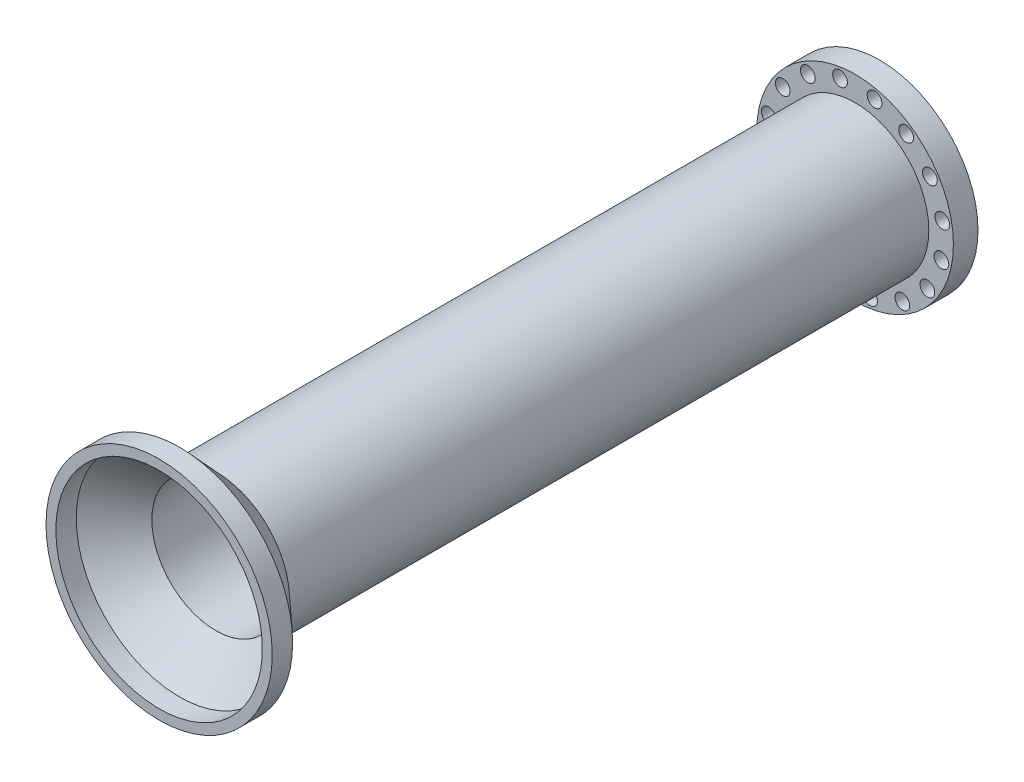
from build123d import *

# Parameters (mm, degrees)
SKETCH1_R               = 20
SKETCH1_R_2             = 15
BOSS_EXTRUDE1_DEPTH     = 5
SKETCH2_R               = 15
BOSS_EXTRUDE2_DEPTH     = 130
CUT_EXTRUDE1_DEPTH      = 160.922689506
CUT_EXTRUDE1_DEPTH_BACK = 130
SKETCH3_R               = 13
SKETCH4_R               = 13
CUT_EXTRUDE2_DEPTH      = 156.724971083
SKETCH11_R              = 1.5
CUT_EXTRUDE4_DEPTH      = 50


with BuildPart() as part:
    # Sketch1 → Boss-Extrude1 (new body)
    # profile 1 of 2: a face of its own
    with BuildSketch(Plane.XY):
        with Locations((20, 55.830512452)):
            Circle(SKETCH1_R)
        with Locations((20, 55.830512452)):
            Circle(SKETCH1_R_2, mode=Mode.SUBTRACT)
    # profile 2 of 2: a face of its own
    with BuildSketch(Plane.XY):
        with Locations((20, 55.830512452)):
            Circle(SKETCH1_R_2)
    extrude(amount=BOSS_EXTRUDE1_DEPTH)

    # Sketch2 → Boss-Extrude2 (add)
    with BuildSketch(Plane.XY.offset(5)):
        with Locations((20, 55.830512452)):
            Circle(SKETCH2_R)
    extrude(amount=BOSS_EXTRUDE2_DEPTH)

    # Sketch3 → Cut-Extrude1 (cut, two sides: drawn at the far end of the back side and taken through both)
    with BuildSketch(Plane.XY.offset(135).offset(-CUT_EXTRUDE1_DEPTH_BACK)):
        with Locations((20, 55.830512452)):
            Circle(SKETCH3_R)
    extrude(amount=CUT_EXTRUDE1_DEPTH + CUT_EXTRUDE1_DEPTH_BACK, mode=Mode.SUBTRACT)

    # Sketch4 → Cut-Extrude2 (cut, through all)
    with BuildSketch(Plane.XY.offset(5)):
        with Locations((20, 55.830512452)):
            Circle(SKETCH4_R)
    extrude(amount=-CUT_EXTRUDE2_DEPTH, mode=Mode.SUBTRACT)

    # Sketch11 → Cut-Extrude4 (cut)
    with BuildSketch(Plane.XY):
        with Locations((10.388397973, 71.049484377)):
            Circle(SKETCH11_R)
        with Locations((16.944086026, 73.569209974)):
            Circle(SKETCH11_R)
        with Locations((23.96500928, 73.388379674)):
            Circle(SKETCH11_R)
        with Locations((30.382295814, 70.534523253)):
            Circle(SKETCH11_R)
        with Locations((35.218971926, 65.442114479)):
            Circle(SKETCH11_R)
        with Locations((37.738697522, 58.886426426)):
            Circle(SKETCH11_R)
        with Locations((37.557867223, 51.865503172)):
            Circle(SKETCH11_R)
        with Locations((34.704010801, 45.448216638)):
            Circle(SKETCH11_R)
        with Locations((29.611602027, 40.611540526)):
            Circle(SKETCH11_R)
        with Locations((23.055913974, 38.09181493)):
            Circle(SKETCH11_R)
        with Locations((16.03499072, 38.272645229)):
            Circle(SKETCH11_R)
        with Locations((9.617704186, 41.126501651)):
            Circle(SKETCH11_R)
        with Locations((4.781028074, 46.218910425)):
            Circle(SKETCH11_R)
        with Locations((2.261302478, 52.774598478)):
            Circle(SKETCH11_R)
        with Locations((2.442132777, 59.795521732)):
            Circle(SKETCH11_R)
        with Locations((5.295989199, 66.212808266)):
            Circle(SKETCH11_R)
    extrude(amount=CUT_EXTRUDE4_DEPTH, mode=Mode.SUBTRACT)


with BuildPart() as body_2:
    # Sketch7 → Revolve1 (revolve)
    with BuildSketch(Plane.ZY.offset(-20), mode=Mode.PRIVATE) as revolve1_sk:
        Polygon((135, 68.830512452), (135, 70.830512452), (142.367477853, 78.830512452), (146.518943946, 78.830512452), (146.518943946, 76.830512452), (142.367477853, 76.830512452), align=None)
    revolve(revolve1_sk.sketch.rotate(Axis((20, 55.830512452, 135), (0, 0, 1)), 90), axis=Axis((20, 55.830512452, 135), (0, 0, 1)))


solid = Compound([part.part, body_2.part])
